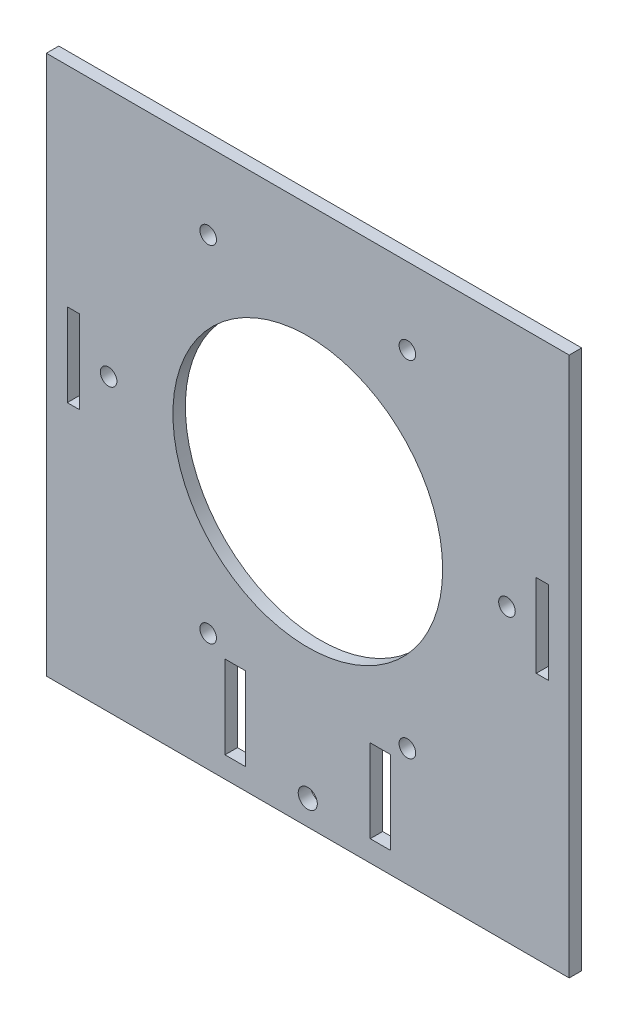
SolidWorks part; units mm, degrees
ref_plane "Front Plane" through (0, 0, 0) normal (0, 0, 1) x (1, 0, 0)
ref_plane "Top Plane" through (0, 0, 0) normal (0, 1, 0) x (1, 0, 0)
ref_plane "Right Plane" through (0, 0, 0) normal (1, 0, 0) x (0, 0, -1)
sketch "Sketch1" plane through (0, 0, 0) normal (0, 0, 1) x (1, 0, 0)
  line L0 (17.5, -44.9) -> (17.5, -64.9) construction
  line L1 (-63, 60) -> (63, 60)
  line L2 (-63, 60) -> (-63, -70)
  line L3 (-63, -70) -> (63, -70)
  line L4 (63, 60) -> (63, -70)
  line L5 (-17.5, -44.9) -> (-17.5, -64.9) construction
  line L15 (-15.05, -44.9) -> (-19.95, -44.9)
  line L16 (-15.05, -44.9) -> (-15.05, -64.9)
  line L17 (-15.05, -64.9) -> (-19.95, -64.9)
  line L18 (-19.95, -44.9) -> (-19.95, -64.9)
  line L22 (0, -70) -> (0, 60) construction
  line L27 (15.05, -44.9) -> (15.05, -64.9)
  line L28 (19.95, -64.9) -> (15.05, -64.9)
  line L29 (19.95, -44.9) -> (19.95, -64.9)
  line L30 (19.95, -44.9) -> (15.05, -44.9)
  circle A0 centre (0, 0) radius 32.5
  dimension "D4" = 63
  dimension "D1" = 65
  dimension "D2" = 35
  dimension "D3" = 4.9
  dimension "D5" = 17.5
  dimension "D6" = 60
  dimension "D7" = 44.9
  dimension "D8" = 64.9
  dimension "D9" = 70
extrude "Boss-Extrude1" add sketch "Sketch1" along normal blind 3
sketch "Sketch2" plane through (0, 0, 3) normal (0, 0, 1) x (1, 0, 0)
  line L0 (-56.5, 9.6) -> (-56.5, -10.4) construction
  line L1 (-57.95, 9.6) -> (-55.05, 9.6)
  line L2 (-57.95, 9.6) -> (-57.95, -10.4)
  line L3 (-57.95, -10.4) -> (-55.05, -10.4)
  line L4 (-55.05, 9.6) -> (-55.05, -10.4)
  line L5 (-63, 60) -> (-63, -70) construction
  line L9 (-63, -70) -> (63, -70) construction
  dimension "D1" = 6.5
  dimension "D2" = 2.9
  dimension "D3" = 59.6
  dimension "D4" = 79.6
extrude "Cut-Extrude1" cut sketch "Sketch2" against normal blind 3
mirror "Mirror1" about plane through (0, 0, 0) normal (1, 0, 0) of "Cut-Extrude1"
hole_wizard "Ø4.0 (4) Diameter Hole1" positions "Sketch5" profile "Sketch4" hole size "Ø4.0" standard "ISO"
sketch "Sketch5" plane through (0, 0, 3) normal (0, 0, 1) x (1, 0, 0)
  point P0 (-24, 41.5692)
  point P3 (48, 0)
  point P6 (24, 41.5692)
  point P9 (24, -41.5692)
  point P12 (-24, -41.5692)
  point P15 (-48, 0)
  dimension "D1" = 24
  dimension "D2" = 48
  dimension "D3" = 24
  dimension "D4" = 48
  dimension "D5" = 41.5692
  dimension "D6" = 41.5692
sketch "Sketch4" plane through (-24, 41.5692, 3) normal (1, 0, 0) x (0, -1, 0)
  line L0 (0, 0) -> (0, 11.2017)
  line L1 (0, 11.2017) -> (2, 10)
  line L2 (2, 10) -> (2, 0)
  line L5 (2, 0) -> (0, 0)
  line L10 (0, 11.2017) -> (-2, 10) construction
  line L11 (0, -6.35) -> (0, 107.95) construction
  dimension "Hole Dia." = 4
  dimension "Hole Depth" = 10
  dimension "Drill Angle" = 118
sketch "Sketch6" plane through (0, 0, 3) normal (0, 0, 1) x (1, 0, 0)
  line L0 (-63, -70) -> (63, -70) construction
  circle A0 centre (0, -64) radius 2.3
  dimension "D1" = 4.6
  dimension "D2" = 6
extrude "Cut-Extrude2" cut sketch "Sketch6" against normal blind 3
